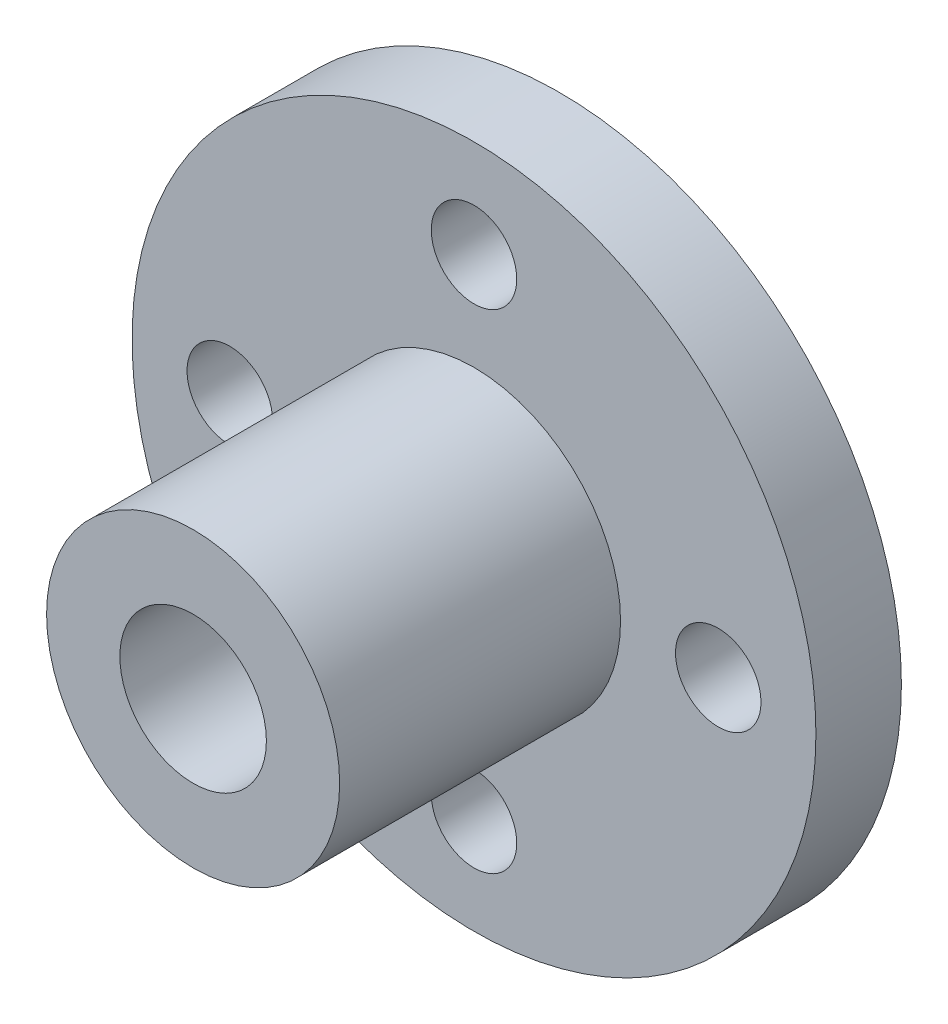
SolidWorks part; units mm, degrees
ref_plane "Front Plane" through (0, 0, 0) normal (0, 0, 1) x (1, 0, 0)
ref_plane "Top Plane" through (0, 0, 0) normal (0, 1, 0) x (1, 0, 0)
ref_plane "Right Plane" through (0, 0, 0) normal (1, 0, 0) x (0, 0, -1)
other "Configuration Table"
sketch "Sketch1" plane through (0, 0, 0) normal (0, 0, 1) x (1, 0, 0)
  circle A0 centre (0, 0) radius 14
  dimension "D1" = 28
extrude "Boss-Extrude1" add sketch "Sketch1" along normal blind 3.5
sketch "Sketch2" plane through (0, 0, 3.5) normal (0, 0, 1) x (1, 0, 0)
  circle A0 centre (0, 0) radius 6
  dimension "D1" = 12
extrude "Boss-Extrude2" add sketch "Sketch2" along normal blind 11.5
sketch "Sketch3" plane through (0, 0, 3.5) normal (0, 0, 1) x (1, 0, 0)
  line L0 (0, 0) -> (0, 10) construction
  circle A0 centre (0, 10) radius 1.75
  dimension "D1" = 3.5
  dimension "D2" = 10
extrude "Cut-Extrude1" cut sketch "Sketch3" against normal blind 11.5
pattern_circular "CirPattern1" count 4 every 90 about axis through (0, 0, 0) along (0, 0, 1) of "Cut-Extrude1"
sketch "Sketch4" plane through (0, 0, 15) normal (0, 0, 1) x (1, 0, 0)
  circle A0 centre (0, 0) radius 3
  dimension "D1" = 6
extrude "Cut-Extrude2" cut sketch "Sketch4" against normal blind 50
